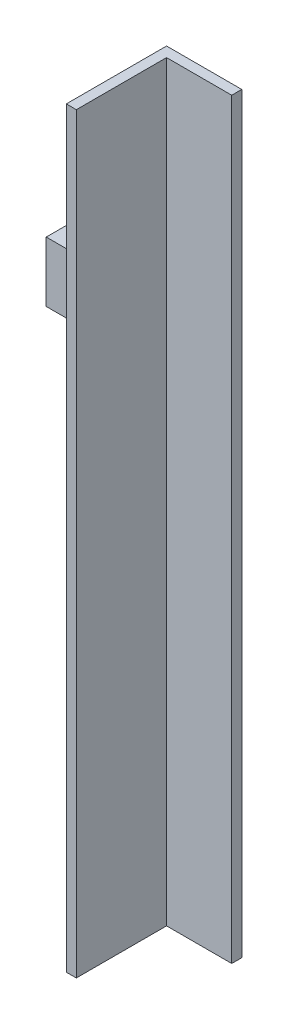
SolidWorks part; units mm, degrees
ref_plane "Front Plane" through (0, 0, 0) normal (0, 0, 1) x (1, 0, 0)
ref_plane "Top Plane" through (0, 0, 0) normal (0, 1, 0) x (1, 0, 0)
ref_plane "Right Plane" through (0, 0, 0) normal (1, 0, 0) x (0, 0, -1)
sketch "Sketch1" plane through (0, 0, 0) normal (0, 0, 1) x (1, 0, 0)
  line L0 (130, 0) -> (100, 0) construction
  line L1 (130, 10) -> (130, -10) construction
  line L2 (100, -3.5) -> (100, 3.5) construction
  line L3 (107.5, 35) -> (92.5, 35)
  line L4 (107.5, 35) -> (107.5, -35)
  line L5 (107.5, -35) -> (92.5, -35)
  line L6 (92.5, 35) -> (92.5, -35)
  line L7 (107.5, 35) -> (92.5, -35) construction
  line L8 (107.5, -35) -> (92.5, 35) construction
  dimension "D1" = 70
  dimension "D2" = 15
extrude "Boss-Extrude1" add sketch "Sketch1" along normal blind 20
sketch "Sketch2" plane through (0, -35, 0) normal (0, -1, 0) x (-1, 0, 0)
  line L0 (-107.5, -2) -> (-94.5, -2)
  line L1 (-107.5, -20) -> (-107.5, 0) construction
  line L2 (-94.5, -2) -> (-94.5, -20)
  line L3 (-92.5, -20) -> (-107.5, -20) construction
  line L4 (-94.5, -20) -> (-107.5, -20)
  line L5 (-107.5, -20) -> (-107.5, -2)
  line L6 (-92.5, 0) -> (-107.5, 0) construction
  line L7 (-92.5, -20) -> (-92.5, 0) construction
  dimension "D1" = 2
  dimension "D2" = 2
extrude "Cut-Extrude1" cut sketch "Sketch2" against normal blind 154
sketch "Sketch3" plane through (0, -35, 0) normal (0, -1, 0) x (1, 0, 0)
  line L6 (107.5, 0) -> (107.5, 2)
  line L7 (107.5, 2) -> (94.5, 2)
  line L8 (94.5, 2) -> (94.5, 20)
  line L9 (94.5, 20) -> (92.5, 20)
  line L10 (92.5, 20) -> (92.5, 0)
  line L11 (92.5, 0) -> (107.5, 0)
  line L12 (107.5, 0) -> (107.5, 2)
  line L13 (107.5, 2) -> (94.5, 2)
  line L14 (94.5, 2) -> (94.5, 20)
  line L15 (94.5, 20) -> (92.5, 20)
  line L16 (92.5, 20) -> (92.5, 0)
  line L17 (92.5, 0) -> (107.5, 0)
  dimension "D1" = 0
extrude "Boss-Extrude2" add sketch "Sketch3" along normal blind 80
sketch "Sketch4" plane through (94.5, 0, 0) normal (1, 0, 0) x (0, 0, -1)
  line L1 (-4, -6) -> (-16, -6)
  line L2 (-4, -6) -> (-4, 6)
  line L3 (-4, 6) -> (-16, 6)
  line L4 (-16, -6) -> (-16, 6)
  line L5 (-4, -6) -> (-16, 6) construction
  line L6 (-4, 6) -> (-16, -6) construction
  circle A0 centre (-10, 0) radius 3.5 construction
  circle A1 centre (-10, 0) radius 3.5
  dimension "D1" = 12
  dimension "D2" = 12
extrude "Boss-Extrude4" add sketch "Sketch4" against normal blind 10
